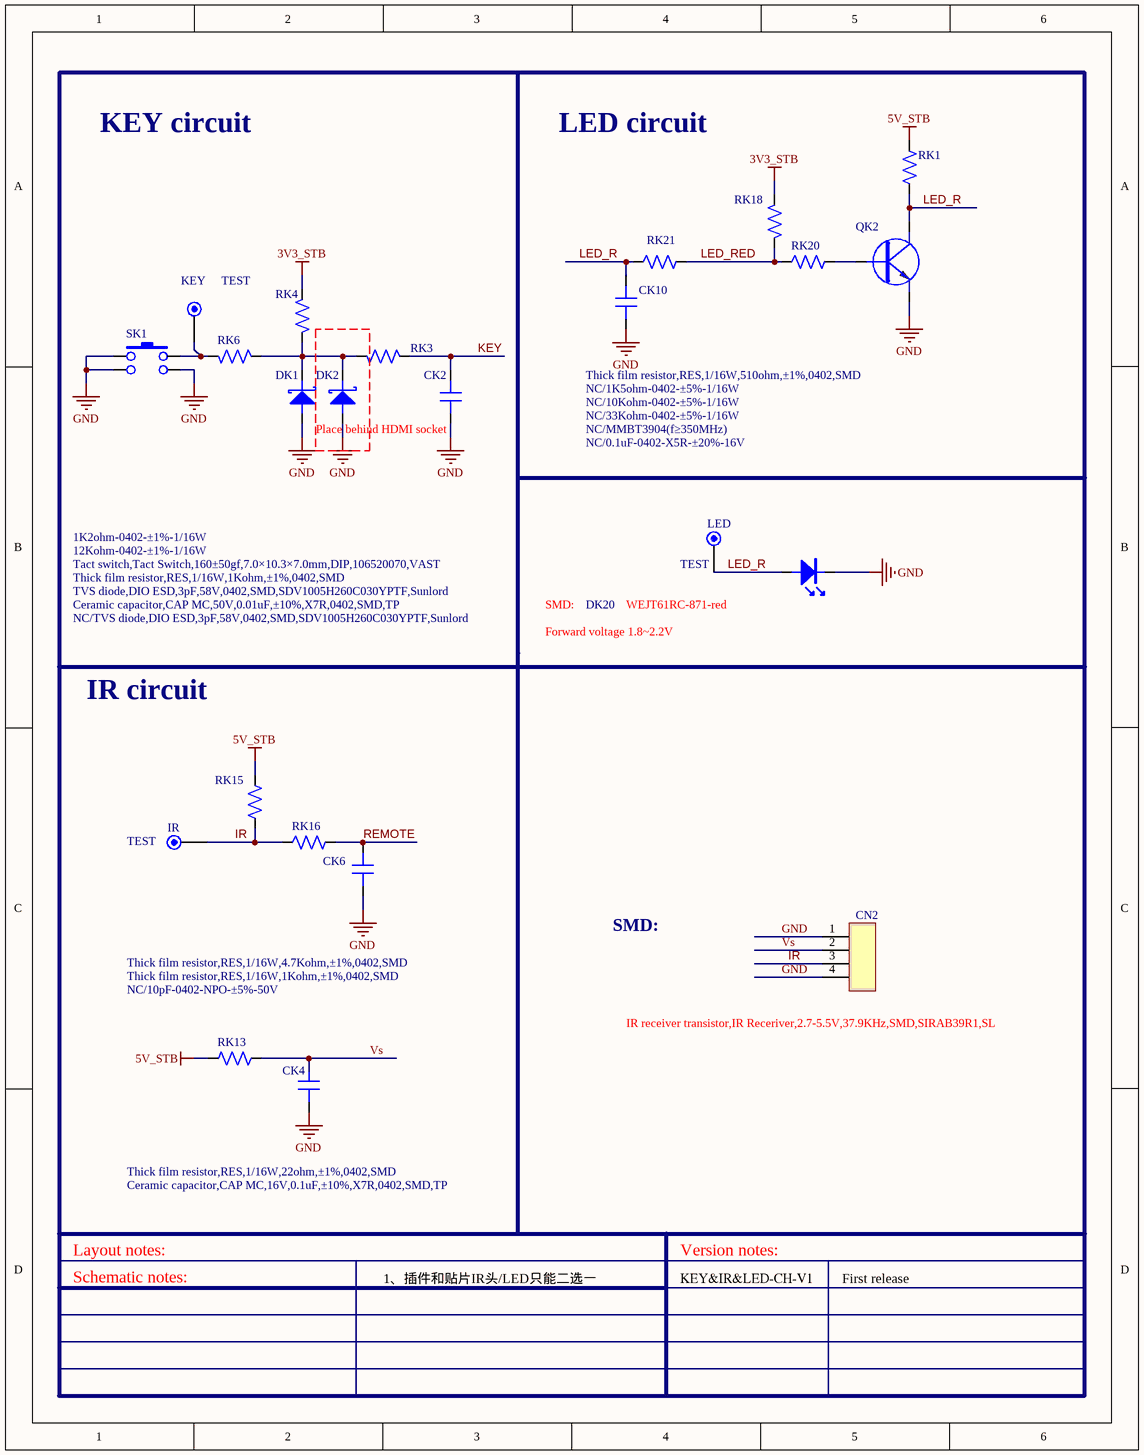
[diagram p0: MISC86383-18.SchDoc]
# Altium project MISC86383-33.PrjPCB (part 5 of 8)

## Sheet MISC86383-18.SchDoc
size 213 x 271 mm

### Parts
CK2  Ceramic capacitor,CAP MC,50V,0.01uF,±10%,X7R,0402,SMD,TP  [C0402]
CK4  Ceramic capacitor,CAP MC,16V,0.1uF,±10%,X7R,0402,SMD,TP  [C0402]
CK6  NC/10pF-0402-NPO-±5%-50V  [C0402]
CK10  NC/0.1uF-0402-X5R-±20%-16V  [C0402]
CN2  IR receiver transistor,IR Receriver,2.7-5.5V,37.9KHz,SMD,SIRAB39R1,SL  [REMOTE-HS-1]
DK1  TVS diode,DIO ESD,3pF,58V,0402,SMD,SDV1005H260C030YPTF,Sunlord  [DIODE-S0402]
DK2  NC/TVS diode,DIO ESD,3pF,58V,0402,SMD,SDV1005H260C030YPTF,Sunlord  [DIODE-S0402]
DK20  WEJT61RC-871-red  [DIODE-S0603]
IR  TEST  [TP]
KEY  TEST  [TP]
LED  TEST  [TP]
QK2  NC/MMBT3904(f≥350MHz)  [SOT-23]
RK1  NC/1K5ohm-0402-±5%-1/16W  [R0402]
RK3  Thick film resistor,RES,1/16W,1Kohm,±1%,0402,SMD  [R0402]
RK4  12Kohm-0402-±1%-1/16W  [R0402]
RK6  1K2ohm-0402-±1%-1/16W  [R0402]
RK13  Thick film resistor,RES,1/16W,22ohm,±1%,0402,SMD  [R0402]
RK15  Thick film resistor,RES,1/16W,4.7Kohm,±1%,0402,SMD  [R0402]
RK16  Thick film resistor,RES,1/16W,1Kohm,±1%,0402,SMD  [R0402]
RK18  NC/33Kohm-0402-±5%-1/16W  [R0402]
RK20  NC/10Kohm-0402-±5%-1/16W  [R0402]
RK21  Thick film resistor,RES,1/16W,510ohm,±1%,0402,SMD  [R0402]
SK1  Tact switch,Tact Switch,160±50gf,7.0×10.3×7.0mm,DIP,106520070,VAST  [KEY-HD-6]

### Blocks framed on the sheet
Place behind HDMI socket: DK2

### Nets
3V3_STB: RK4.2 RK18.2
5V_STB: RK1.2 RK13.1 RK15.1
GND: CK2.2 CK4.2 CK6.1 CK10.1 CN2.1 CN2.4 DK1.A DK2.A DK20.K QK2.E SK1.1 SK1.3 SK1.4
IR: CN2.3 IR.1 RK15.2 RK16.2
KEY: CK2.1 RK3.1
LED_R: CK10.2 DK20.A LED.1 QK2.C RK1.1 RK21.2
LED_RED: RK18.1 RK20.2 RK21.1
REMOTE: CK6.2 RK16.1
Vs: CK4.1 CN2.2 RK13.2
NetDK1_K: DK1.K DK2.K RK3.2 RK4.1 RK6.1
NetKEY_1: KEY.1 RK6.2 SK1.2
NetQK2_B: QK2.B RK20.1

### Notes on the sheet
- KEY circuit
- LED circuit
- SMD:
- Forward voltage 1.8~2.2V
- IR circuit
- Layout notes:
- Version notes:
- Schematic notes:
- 1、插件和贴片IR头/LED只能二选一
- KEY&IR&LED-CH-V1
- First release

### Library data of the parts
CK2 = 0.01uF-0402-X7R-±10%-50V-D
CK4 CK10 = 0.1uF-0402-Y5V-+80%-20%-16V-D
CK6 = 10pF-0402-NPO-±5%-50V-D
CN2 = 红外接收三极管,Phototransistor,NPN,6.8×3×3.2mm,SMD,HS75438D,VISHAY-D
DK1 DK2 = AVLC18S02003-D
DK20 = WEJT61RC-871-红色-D
QK2 = MMBT3904(f≥350MHz)-D-NPN: Q-NPN-#-#-#
RK1 = 22ohm-0402-±5%-1/16W-D
RK3 RK16 RK21 = 1Kohm-0402-±5%-1/16W-D
RK4 RK6 = 4K7ohm-0402-±1%-1/16W-D
RK13 = 100ohm-0402-±5%-1/16W-D
RK15 RK18 = 4K7ohm-0402-±5%-1/16W-D
RK20 = 10Kohm-0402-±5%-1/16W-D
SK1 = 轻触开关,Tact Switch,160±50gf,7.0×10.3×7.0mm,DIP,KFC-A06-E-4-7.5/4(R),YK-DLMI